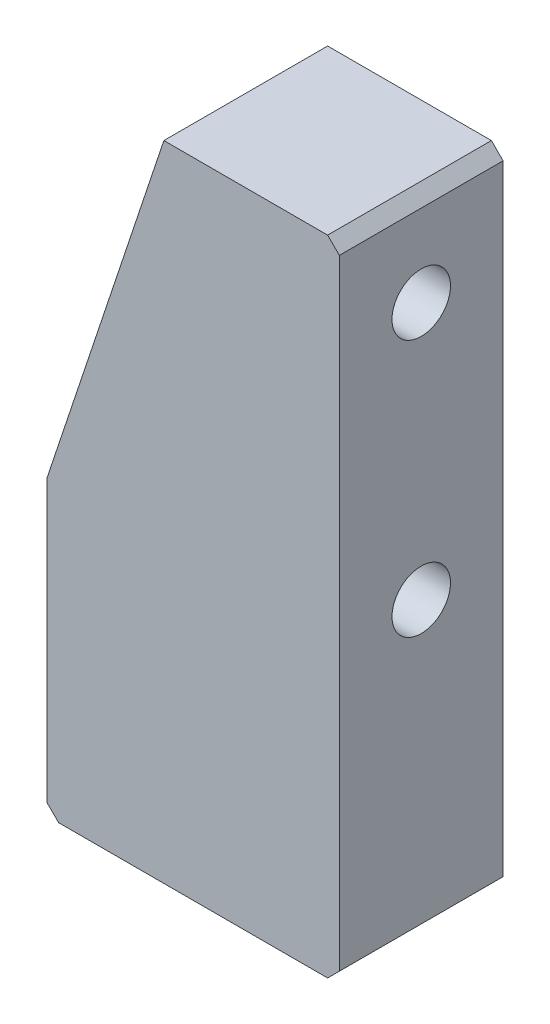
from build123d import *

# Parameters (mm, degrees)
BOSS_EXTRUDE2_DEPTH   = 7
M6_TAPPED_HOLE1_D     = 5
M6_TAPPED_HOLE1_DEPTH = 15
M6_TAPPED_HOLE1_TIP   = 1.502151548
M6_TAPPED_HOLE2_D     = 5
M6_TAPPED_HOLE2_DEPTH = 15
M6_TAPPED_HOLE2_TIP   = 1.502151548
CHAMFER1_SIZE         = 1


with BuildPart() as part:
    # Sketch6 → Boss-Extrude2 (new, symmetric)
    with BuildSketch(Plane.XY):
        Polygon((0, 0), (0, 55), (-15, 55), (-25, 25), (-25, 0), align=None)
    extrude(amount=BOSS_EXTRUDE2_DEPTH, both=True)

    # M6 Tapped Hole1
    with Locations(Plane(origin=(0, 0, 0), x_dir=(0, 0, -1), z_dir=(1, 0, 0))):
        with Locations((0, 25), (0, 47)):
            Hole(M6_TAPPED_HOLE1_D / 2, depth=M6_TAPPED_HOLE1_DEPTH)
            with Locations((0, 0, -(M6_TAPPED_HOLE1_DEPTH + M6_TAPPED_HOLE1_TIP / 2))):  # 118° drill point
                Cone(0, M6_TAPPED_HOLE1_D / 2, M6_TAPPED_HOLE1_TIP, mode=Mode.SUBTRACT)

    # M6 Tapped Hole2
    with Locations(Plane(origin=(0, 0, 0), x_dir=(-1, 0, 0), z_dir=(0, -1, 0))):
        with Locations((16, 0)):
            Hole(M6_TAPPED_HOLE2_D / 2, depth=M6_TAPPED_HOLE2_DEPTH)
            with Locations((0, 0, -(M6_TAPPED_HOLE2_DEPTH + M6_TAPPED_HOLE2_TIP / 2))):  # 118° drill point
                Cone(0, M6_TAPPED_HOLE2_D / 2, M6_TAPPED_HOLE2_TIP, mode=Mode.SUBTRACT)

    # Chamfer1
    chamfer1_edges = [part.edges().sort_by_distance(p)[0] for p in [
        (-25, 0, 0),
        (0, 55, 0),
        (0, 0, 0),
    ]]
    chamfer(chamfer1_edges, length=CHAMFER1_SIZE)


solid = part.part
